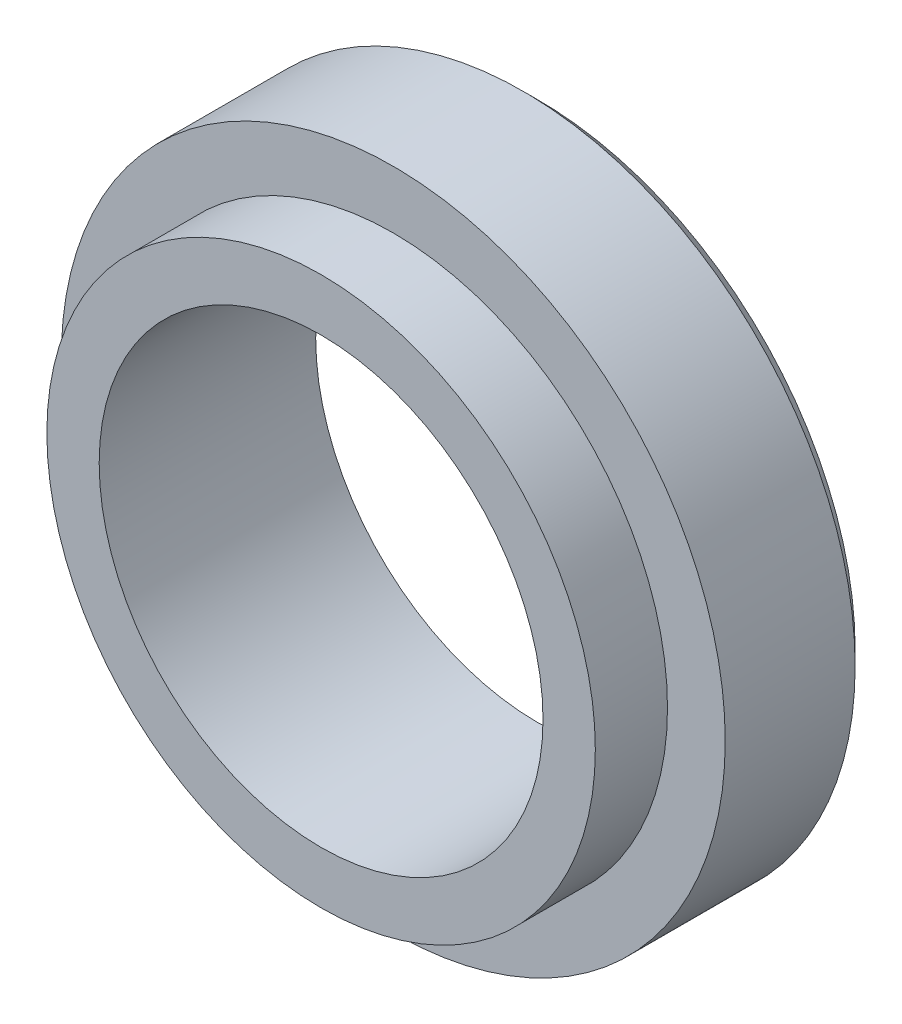
from build123d import *

# Parameters (mm, degrees)
SKETCH1_R             = 19
SKETCH1_R_2           = 7.5
BOSS_EXTRUDE1_DEPTH   = 10
SKETCH2_R             = 23
SKETCH2_R_2           = 7.5
BOSS_EXTRUDE2_DEPTH   = 10
SKETCH3_R             = 19
SKETCH3_R_2           = 7.5
BOSS_EXTRUDE3_DEPTH   = 5
G1_TAPPED_HOLE1_D     = 30.75
G1_TAPPED_HOLE1_DEPTH = 73.43
G1_TAPPED_HOLE1_TIP   = 9.238232018
SKETCH6_R             = 28.473904373
CUT_EXTRUDE1_DEPTH    = 10
CHAMFER2_SIZE         = 1


with BuildPart() as part:
    # Sketch1 → Boss-Extrude1 (new body)
    with BuildSketch(Plane.XY):
        Circle(SKETCH1_R)
        Circle(SKETCH1_R_2, mode=Mode.SUBTRACT)
    extrude(amount=BOSS_EXTRUDE1_DEPTH)

    # Sketch2 → Boss-Extrude2 (add)
    with BuildSketch(Plane.XY.offset(10)):
        Circle(SKETCH2_R)
        Circle(SKETCH2_R_2, mode=Mode.SUBTRACT)
    extrude(amount=BOSS_EXTRUDE2_DEPTH)

    # Sketch3 → Boss-Extrude3 (add)
    with BuildSketch(Plane.XY.offset(20)):
        Circle(SKETCH3_R)
        Circle(SKETCH3_R_2, mode=Mode.SUBTRACT)
    extrude(amount=BOSS_EXTRUDE3_DEPTH)

    # G1 Tapped Hole1
    with Locations(Plane.XY.offset(25)):
        with Locations((0, 0)):
            Hole(G1_TAPPED_HOLE1_D / 2, depth=G1_TAPPED_HOLE1_DEPTH)
            with Locations((0, 0, -(G1_TAPPED_HOLE1_DEPTH + G1_TAPPED_HOLE1_TIP / 2))):  # 118° drill point
                Cone(0, G1_TAPPED_HOLE1_D / 2, G1_TAPPED_HOLE1_TIP, mode=Mode.SUBTRACT)

    # Sketch6 → Cut-Extrude1 (cut)
    with BuildSketch(Plane.XY):
        Circle(SKETCH6_R)
    extrude(amount=CUT_EXTRUDE1_DEPTH, mode=Mode.SUBTRACT)

    # Chamfer2
    chamfer2_edges = [part.edges().sort_by_distance(p)[0] for p in [
        (-23, 0, 10),
    ]]
    chamfer(chamfer2_edges, length=CHAMFER2_SIZE)


solid = part.part
